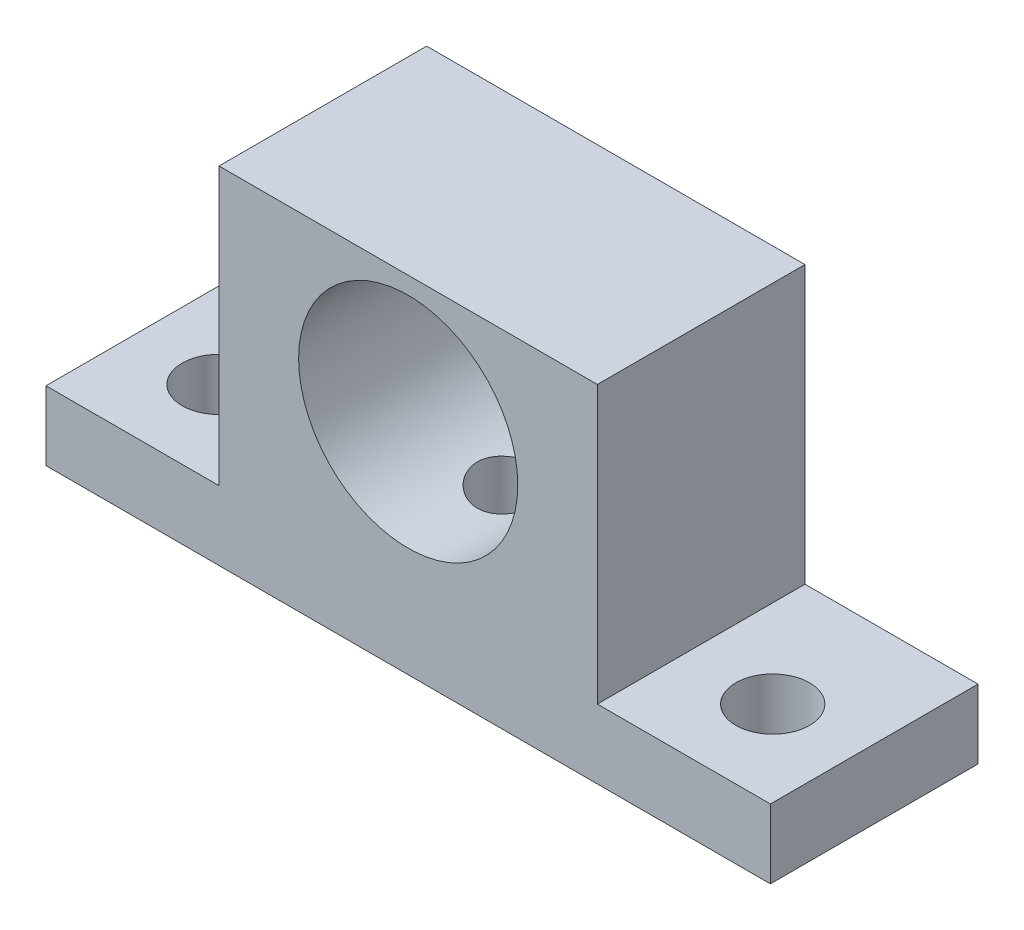
SolidWorks part; units mm, degrees
ref_plane "Front Plane" through (0, 0, 0) normal (0, 0, 1) x (1, 0, 0)
ref_plane "Top Plane" through (0, 0, 0) normal (0, 1, 0) x (1, 0, 0)
ref_plane "Right Plane" through (0, 0, 0) normal (1, 0, 0) x (0, 0, -1)
sketch "Sketch1" plane through (0, 0, 0) normal (0, 1, 0) x (1, 0, 0)
  line L1 (0, 0) -> (40.4, 0)
  line L2 (0, 0) -> (0, -20)
  line L3 (0, -20) -> (40.4, -20)
  line L4 (40.4, 0) -> (40.4, -20)
extrude "Boss-Extrude1" add sketch "Sketch1" along normal blind 15
sketch "Sketch2" plane through (0, 0, 20) normal (0, 0, 1) x (1, 0, 0)
  line L0 (20.2, 15) -> (20.2, 0) construction
  line L1 (0, 15) -> (40.4, 15) construction
  line L2 (0, 0) -> (40.4, 0) construction
  circle A0 centre (20.2, 9.5) radius 4.75
  dimension "D1" = 9.5
extrude "Cut-Extrude1" cut sketch "Sketch2" against normal blind 36
sketch "Sketch3" plane through (0, 15, 0) normal (0, 1, 0) x (1, 0, 0)
  line L0 (0, 0) -> (0, -20) construction
  line L1 (20.2, 0) -> (20.2, -20) construction
  line L2 (40.4, 0) -> (0, 0) construction
  line L3 (0, -20) -> (40.4, -20) construction
  circle A0 centre (8.2, -14) radius 1.6
  circle A1 centre (32.2, -14) radius 1.6
  dimension "D1" = 8.2
  dimension "D2" = 6
extrude "Cut-Extrude2" cut sketch "Sketch3" against normal blind 36
sketch "Sketch4" plane through (0, 15, 0) normal (0, 1, 0) x (1, 0, 0)
  line L0 (0, 0) -> (0, -20) construction
  line L1 (40.4, 0) -> (0, 0)
  line L2 (40.4, 0) -> (40.4, -8.8)
  line L3 (40.4, -8.8) -> (0, -8.8)
  line L4 (0, 0) -> (0, -8.8)
  line L5 (0, -20) -> (40.4, -20) construction
  dimension "D1" = 11.2
extrude "Cut-Extrude3" cut sketch "Sketch4" against normal blind 36
sketch "Sketch5" plane through (0, 15, 0) normal (0, 1, 0) x (1, 0, 0)
  line L0 (40.4, -20) -> (40.4, -8.8) construction
  line L1 (0, -20) -> (40.4, -20)
  line L2 (0, -20) -> (0, -17.8)
  line L3 (0, -17.8) -> (40.4, -17.8)
  line L4 (40.4, -20) -> (40.4, -17.8)
  line L5 (0, -8.8) -> (40.4, -8.8) construction
  dimension "D1" = 9
extrude "Cut-Extrude4" cut sketch "Sketch5" against normal blind 36
sketch "Sketch8" plane through (0, 15, 0) normal (0, 1, 0) x (1, 0, 0)
  line L0 (40.4, -17.8) -> (0, -17.8) construction
  line L1 (0, -8.8) -> (12, -8.8)
  line L2 (0, -8.8) -> (0, -17.8)
  line L3 (0, -17.8) -> (12, -17.8)
  line L4 (12, -8.8) -> (12, -17.8)
  line L5 (0, -8.8) -> (40.4, -8.8) construction
  line L6 (40.4, -17.8) -> (28.4, -17.8)
  line L7 (40.4, -17.8) -> (40.4, -8.8)
  line L8 (40.4, -8.8) -> (28.4, -8.8)
  line L9 (28.4, -17.8) -> (28.4, -8.8)
extrude "Cut-Extrude6" cut sketch "Sketch8" against normal blind 12
sketch "Sketch10" plane through (0, 3, 0) normal (0, 1, 0) x (1, 0, 0)
  line L0 (0, -17.8) -> (12, -17.8) construction
  line L1 (0, -8.8) -> (4.5, -8.8)
  line L2 (0, -8.8) -> (0, -17.8)
  line L3 (0, -17.8) -> (4.5, -17.8)
  line L4 (4.5, -8.8) -> (4.5, -17.8)
  line L5 (40.4, -8.8) -> (28.4, -8.8) construction
  line L6 (40.4, -17.8) -> (35.9, -17.8)
  line L7 (40.4, -17.8) -> (40.4, -8.8)
  line L8 (40.4, -8.8) -> (35.9, -8.8)
  line L9 (35.9, -17.8) -> (35.9, -8.8)
extrude "Cut-Extrude7" cut sketch "Sketch10" against normal blind 12
sketch "Sketch11" plane through (0, 0, 0) normal (0, -1, 0) x (1, 0, 0)
  circle A0 centre (20.2, 13.3) radius 1.5
extrude "Cut-Extrude8" cut sketch "Sketch11" against normal blind 10
